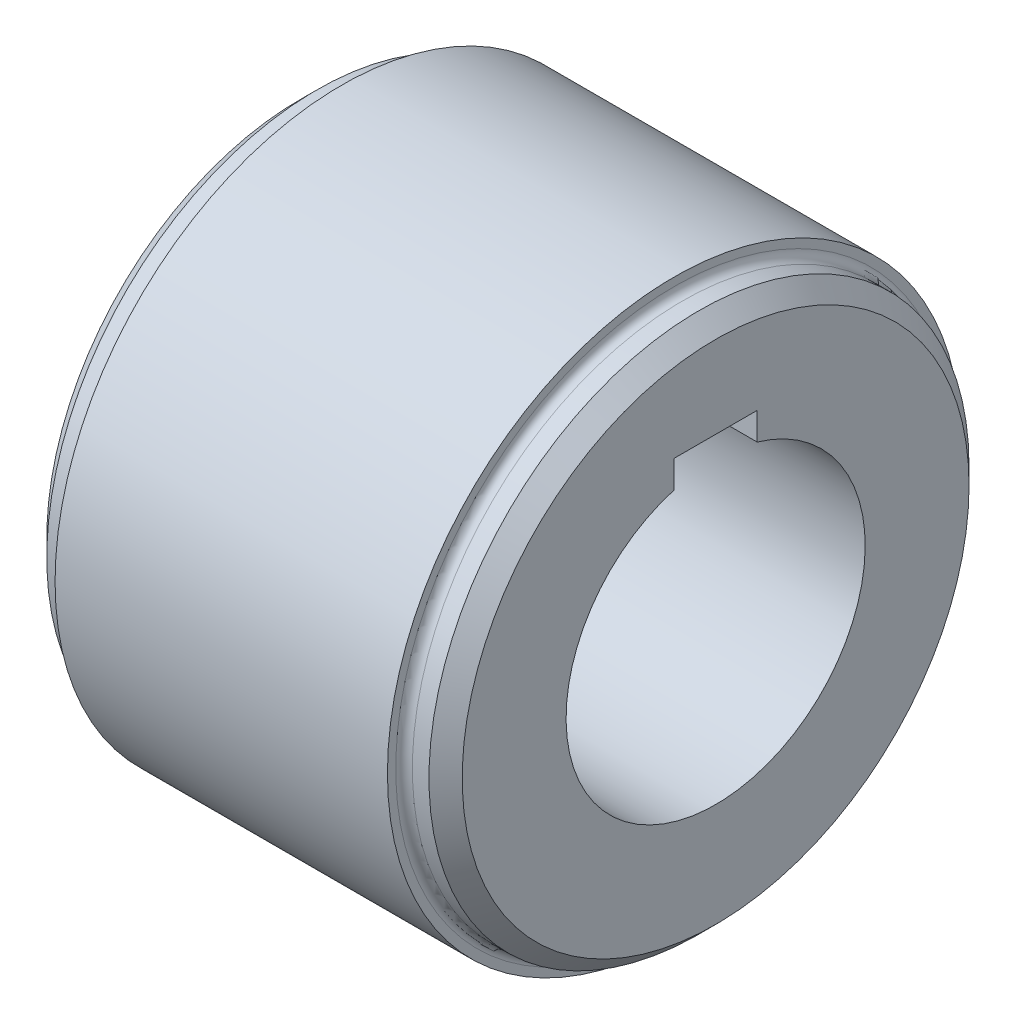
from build123d import *

# Parameters (mm, degrees)
SKETCH_1_R      = 32.5
EXTRUDE_1_DEPTH = 25
SKETCH_2_R      = 34.5
SKETCH_2_R_2    = 32.5
EXTRUDE_2_DEPTH = 20
FILLET_1_R      = 1
CHAMFER_1_SIZE  = 2


with BuildPart() as part:
    # 草图1 → 凸台-拉伸1 (new, symmetric)
    with BuildSketch(Plane(origin=(0, 0, 0), x_dir=(0, 0, -1), z_dir=(1, 0, 0))):
        Circle(SKETCH_1_R)
        with BuildLine():
            Line((5, 17.291616466), (5, 20.591616466))
            Line((5, 20.591616466), (-5, 20.591616466))
            Line((-5, 20.591616466), (-5, 17.291616466))
            ThreePointArc((-5, 17.291616466), (0, -18), (5, 17.291616466))
        make_face(mode=Mode.SUBTRACT)
    extrude(amount=EXTRUDE_1_DEPTH, both=True)

    # 草图2 → 凸台-拉伸2 (add, symmetric)
    with BuildSketch(Plane(origin=(0, 0, 0), x_dir=(0, 0, -1), z_dir=(1, 0, 0))):
        Circle(SKETCH_2_R)
        Circle(SKETCH_2_R_2, mode=Mode.SUBTRACT)
    extrude(amount=EXTRUDE_2_DEPTH, both=True)

    # 圆角1
    fillet_1_edges = [part.edges().sort_by_distance(p)[0] for p in [
        (-20, 0, 32.5),
        (20, 0, 32.5),
    ]]
    fillet(fillet_1_edges, radius=FILLET_1_R)

    # 倒角1
    chamfer_1_edges = [part.edges().sort_by_distance(p)[0] for p in [
        (-25, 0, 32.5),
        (25, 0, 32.5),
    ]]
    chamfer(chamfer_1_edges, length=CHAMFER_1_SIZE)


solid = part.part
